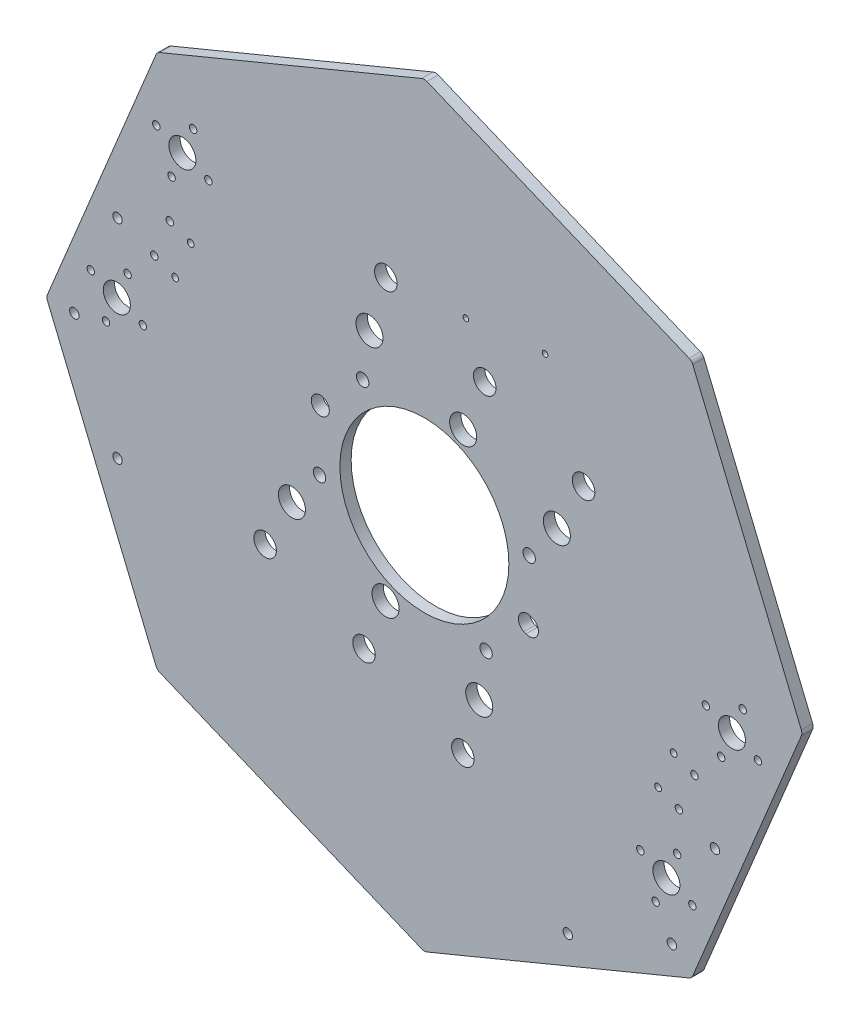
from build123d import *

# Parameters (mm, degrees)
BOSS_EXTRUDE1_DEPTH      = 5
SKETCH2_R                = 37.5
CUT_EXTRUDE1_DEPTH       = 10
SKETCH3_R                = 1
CUT_EXTRUDE2_DEPTH       = 10
M5_TAPPED_HOLE1_D        = 4.2
M5_TAPPED_HOLE1_DEPTH    = 12.4
M5_TAPPED_HOLE1_TIP      = 1.2618073
SKETCH5_R                = 2.75
CUT_EXTRUDE3_DEPTH       = 10
SKETCH6_R                = 5
CUT_EXTRUDE4_DEPTH       = 55
SKETCH7_R                = 4
CUT_EXTRUDE5_DEPTH       = 15
SKETCH8_R                = 6
CUT_EXTRUDE6_DEPTH       = 10
SKETCH9_R                = 6
CUT_EXTRUDE7_DEPTH       = 10
SKETCH10_R               = 1
CUT_EXTRUDE8_DEPTH       = 10
M4_TAPPED_HOLE1_D        = 3.3
M4_TAPPED_HOLE1_DEPTH    = 10.1
M4_TAPPED_HOLE1_TIP      = 0.991420021
M4_TAPPED_HOLE2_D        = 3.3
F_3_0_3_DIAMETER_HOLE1_D = 3
M3_TAPPED_HOLE1_D        = 2.5
FILLET1_R                = 3
CUT_EXTRUDE9_DEPTH       = 237.966923416


with BuildPart() as part:
    # Sketch1 → Boss-Extrude1 (new body)
    with BuildSketch(Plane.XY):
        Polygon((-167.770791045, 0), (-118.631864033, -118.631864033), (0, -167.770791045), (118.631864033, -118.631864033), (167.770791045, 0), (118.631864033, 118.631864033), (0, 167.770791045), (-118.631864033, 118.631864033), align=None)
    extrude(amount=BOSS_EXTRUDE1_DEPTH)

    # Sketch2 → Cut-Extrude1 (cut)
    with BuildSketch(Plane(origin=(0, 0, 0), x_dir=(-1, 0, 0), z_dir=(0, 0, -1))):
        Circle(SKETCH2_R)
    extrude(amount=-CUT_EXTRUDE1_DEPTH, mode=Mode.SUBTRACT)

    # Sketch3 → Cut-Extrude2 (cut)
    with BuildSketch(Plane.XY.offset(5)):
        with Locations((-136.189109124, 46.193976626)):
            Circle(SKETCH3_R)
        with Locations((-155.323280742, 0)):
            Circle(SKETCH3_R)
        with Locations((-136.189109124, -46.193976626)):
            Circle(SKETCH3_R)
        with Locations((63.636168463, -128.964316707)):
            Circle(SKETCH3_R)
        with Locations((109.830145089, -109.830145089)):
            Circle(SKETCH3_R)
        with Locations((128.964316707, -63.636168463)):
            Circle(SKETCH3_R)
    extrude(amount=-CUT_EXTRUDE2_DEPTH, mode=Mode.SUBTRACT)

    # M5 Tapped Hole1
    with Locations(Plane(origin=(-136.189109124, 46.193976626, 0), x_dir=(-1, 0, 0), z_dir=(0, 0, -1))):
        with Locations((0, 0), (19.134171618, -46.193976626), (-246.019254213, -156.024121715), (-265.153425831, -109.830145089), (-199.825277587, -175.158293333), (0, -92.387953252)):
            Hole(M5_TAPPED_HOLE1_D / 2, depth=M5_TAPPED_HOLE1_DEPTH)
            with Locations((0, 0, -(M5_TAPPED_HOLE1_DEPTH + M5_TAPPED_HOLE1_TIP / 2))):  # 118° drill point
                Cone(0, M5_TAPPED_HOLE1_D / 2, M5_TAPPED_HOLE1_TIP, mode=Mode.SUBTRACT)

    # Sketch5 → Cut-Extrude3 (cut)
    with BuildSketch(Plane(origin=(0, 0, 0), x_dir=(-1, 0, 0), z_dir=(0, 0, -1))):
        with Locations((-27.388095491, -38.404325607)):
            Circle(SKETCH5_R)
        with Locations(Location((46.52226711, -7.789651018, 0), (0, 0, 180))):
            Circle(SKETCH5_R)
        with Locations((27.388095491, 38.404325607)):
            Circle(SKETCH5_R)
        with Locations(Location((-46.52226711, 7.789651018, 0), (0, 0, 180))):
            Circle(SKETCH5_R)
    extrude(amount=-CUT_EXTRUDE3_DEPTH, mode=Mode.SUBTRACT)

    # Sketch6 → Cut-Extrude4 (cut)
    with BuildSketch(Plane(origin=(0, 0, 0), x_dir=(-1, 0, 0), z_dir=(0, 0, -1))):
        with Locations((-70.67211806, 46.494104238)):
            Circle(SKETCH6_R)
        with Locations((-26.787840266, 64.671567276)):
            Circle(SKETCH6_R)
        with Locations(Location((17.096437529, 82.849030313, 0), (0, 0, 180))):
            Circle(SKETCH6_R)
        with Locations((70.67211806, -46.494104238)):
            Circle(SKETCH6_R)
        with Locations(Location((26.787840266, -64.671567276, 0), (0, 0, 180))):
            Circle(SKETCH6_R)
        with Locations(Location((-17.096437529, -82.849030313, 0), (0, 0, 180))):
            Circle(SKETCH6_R)
    extrude(amount=-CUT_EXTRUDE4_DEPTH, mode=Mode.SUBTRACT)

    # Sketch7 → Cut-Extrude5 (cut)
    with BuildSketch(Plane.XY.offset(5)):
        with Locations((46.193976626, -19.134171618)):
            Circle(SKETCH7_R)
        with Locations((-46.193976626, 19.134171618)):
            Circle(SKETCH7_R)
    extrude(amount=-CUT_EXTRUDE5_DEPTH, mode=Mode.SUBTRACT)

    # Sketch8 → Cut-Extrude6 (cut)
    with BuildSketch(Plane(origin=(0, 0, 0), x_dir=(-1, 0, 0), z_dir=(0, 0, -1))):
        with Locations((-58.795333419, 24.353824507)):
            Circle(SKETCH8_R)
        with Locations((-17.220754456, 41.574578963)):
            Circle(SKETCH8_R)
        with Locations(Location((24.353824507, 58.795333419, 0), (0, 0, 180))):
            Circle(SKETCH8_R)
        with Locations((58.795333419, -24.353824507)):
            Circle(SKETCH8_R)
        with Locations(Location((17.220754456, -41.574578963, 0), (0, 0, 180))):
            Circle(SKETCH8_R)
        with Locations(Location((-24.353824507, -58.795333419, 0), (0, 0, 180))):
            Circle(SKETCH8_R)
    extrude(amount=-CUT_EXTRUDE6_DEPTH, mode=Mode.SUBTRACT)

    # Sketch9 → Cut-Extrude7 (cut)
    with BuildSketch(Plane(origin=(0, 0, 0), x_dir=(-1, 0, 0), z_dir=(0, 0, -1))):
        with Locations((-136.494068721, -15.406790837)):
            Circle(SKETCH9_R)
        with Locations(Location((-107.410127862, -85.621635308, 0), (0, 0, 180))):
            Circle(SKETCH9_R)
        with Locations((136.494068721, 15.406790837)):
            Circle(SKETCH9_R)
        with Locations(Location((107.410127862, 85.621635308, 0), (0, 0, 180))):
            Circle(SKETCH9_R)
    extrude(amount=-CUT_EXTRUDE7_DEPTH, mode=Mode.SUBTRACT)

    # Sketch10 → Cut-Extrude8 (cut)
    with BuildSketch(Plane(origin=(0, 0, 0), x_dir=(-1, 0, 0), z_dir=(0, 0, -1))):
        with Locations((-141.277611626, -3.85829668)):
            Circle(SKETCH10_R)
        with Locations(Location((-131.710525817, -26.955284993, 0), (0, 0, 180))):
            Circle(SKETCH10_R)
        with Locations((-148.042562878, -20.190333741)):
            Circle(SKETCH10_R)
        with Locations(Location((-124.945574565, -10.623247932, 0), (0, 0, 180))):
            Circle(SKETCH10_R)
        with Locations(Location((-118.958622018, -90.405178212, 0), (0, 0, 180))):
            Circle(SKETCH10_R)
        with Locations((-112.193670766, -74.073141151)):
            Circle(SKETCH10_R)
        with Locations((-95.861633705, -80.838092403)):
            Circle(SKETCH10_R)
        with Locations(Location((-102.626584957, -97.170129464, 0), (0, 0, 180))):
            Circle(SKETCH10_R)
        with Locations((148.042562878, 20.190333741)):
            Circle(SKETCH10_R)
        with Locations(Location((131.710525817, 26.955284993, 0), (0, 0, 180))):
            Circle(SKETCH10_R)
        with Locations(Location((124.945574565, 10.623247932, 0), (0, 0, 180))):
            Circle(SKETCH10_R)
        with Locations((141.277611626, 3.85829668)):
            Circle(SKETCH10_R)
        with Locations(Location((118.958622018, 90.405178212, 0), (0, 0, 180))):
            Circle(SKETCH10_R)
        with Locations((95.861633705, 80.838092403)):
            Circle(SKETCH10_R)
        with Locations(Location((102.626584957, 97.170129464, 0), (0, 0, 180))):
            Circle(SKETCH10_R)
        with Locations((112.193670766, 74.073141151)):
            Circle(SKETCH10_R)
    extrude(amount=-CUT_EXTRUDE8_DEPTH, mode=Mode.SUBTRACT)

    # M4 Tapped Hole1
    with Locations(Plane(origin=(141.277611626, -3.85829668, 0), x_dir=(-1, 0, 0), z_dir=(0, 0, -1))):
        with Locations((0, 0), (-6.764951252, -16.332037061), (16.332037061, -6.764951252), (9.567085809, -23.096988313), (29.08394086, -70.214844471), (22.318989608, -86.546881532), (38.651026669, -93.311832784), (45.415977921, -76.979795723), (282.555223252, 7.71659336), (289.320174504, 24.048630421), (272.988137443, 30.813581673), (266.223186191, 14.481544612), (243.904196583, 101.028426144), (253.471282392, 77.931437831), (260.236233644, 94.263474892), (237.139245331, 84.696389083)):
            Hole(M4_TAPPED_HOLE1_D / 2, depth=M4_TAPPED_HOLE1_DEPTH)
            with Locations((0, 0, -(M4_TAPPED_HOLE1_DEPTH + M4_TAPPED_HOLE1_TIP / 2))):  # 118° drill point
                Cone(0, M4_TAPPED_HOLE1_D / 2, M4_TAPPED_HOLE1_TIP, mode=Mode.SUBTRACT)

    # M4 Tapped Hole2 (through all)
    with Locations(Plane.XY.offset(5)):
        with Locations((-112.964670205, 56.533028271), (-119.852971988, 39.903196685), (119.852971988, -39.903196685), (112.964670205, -56.533028271)):
            Hole(M4_TAPPED_HOLE2_D / 2)

    # Ø3.0 (3) Diameter Hole1 (through all)
    with Locations(Plane.XY.offset(5)):
        with Locations((110.614176663, -36.076362362), (103.72587488, -52.706193947), (-103.72587488, 52.706193947), (-110.614176663, 36.076362362)):
            Hole(F_3_0_3_DIAMETER_HOLE1_D / 2)

    # M3 Tapped Hole1 (through all)
    with Locations(Plane(origin=(0, 0, 0), x_dir=(-1, 0, 0), z_dir=(0, 0, -1))):
        with Locations((-18.399300713, 84.923293231), (-53.561047521, 88.804355428)):
            Hole(M3_TAPPED_HOLE1_D / 2)

    # Fillet1
    fillet1_edges = [part.edges().sort_by_distance(p)[0] for p in [
        (-118.631864033, -118.631864033, 2.5),
        (-167.770791045, 0, 2.5),
        (-118.631864033, 118.631864033, 2.5),
        (0, 167.770791045, 2.5),
        (118.631864033, 118.631864033, 2.5),
        (167.770791045, 0, 2.5),
        (118.631864033, -118.631864033, 2.5),
        (0, -167.770791045, 2.5),
    ]]
    fillet(fillet1_edges, radius=FILLET1_R)

    # Sketch20 → Cut-Extrude9 (cut, through all)
    with BuildSketch(Plane.XY.offset(5)):
        with BuildLine():
            Line((47.262770589, -15.247311772), (48.186650121, -15.629995204))
            ThreePointArc((48.186650121, -15.629995204), (50.351434522, -20.856247064), (45.125182662, -23.021031464))
            Line((45.125182662, -23.021031464), (44.20130313, -22.638348032))
            ThreePointArc((44.20130313, -22.638348032), (42.036518729, -17.412096173), (47.262770589, -15.247311772))
        make_face()
    extrude(amount=-CUT_EXTRUDE9_DEPTH, mode=Mode.SUBTRACT)


solid = part.part
